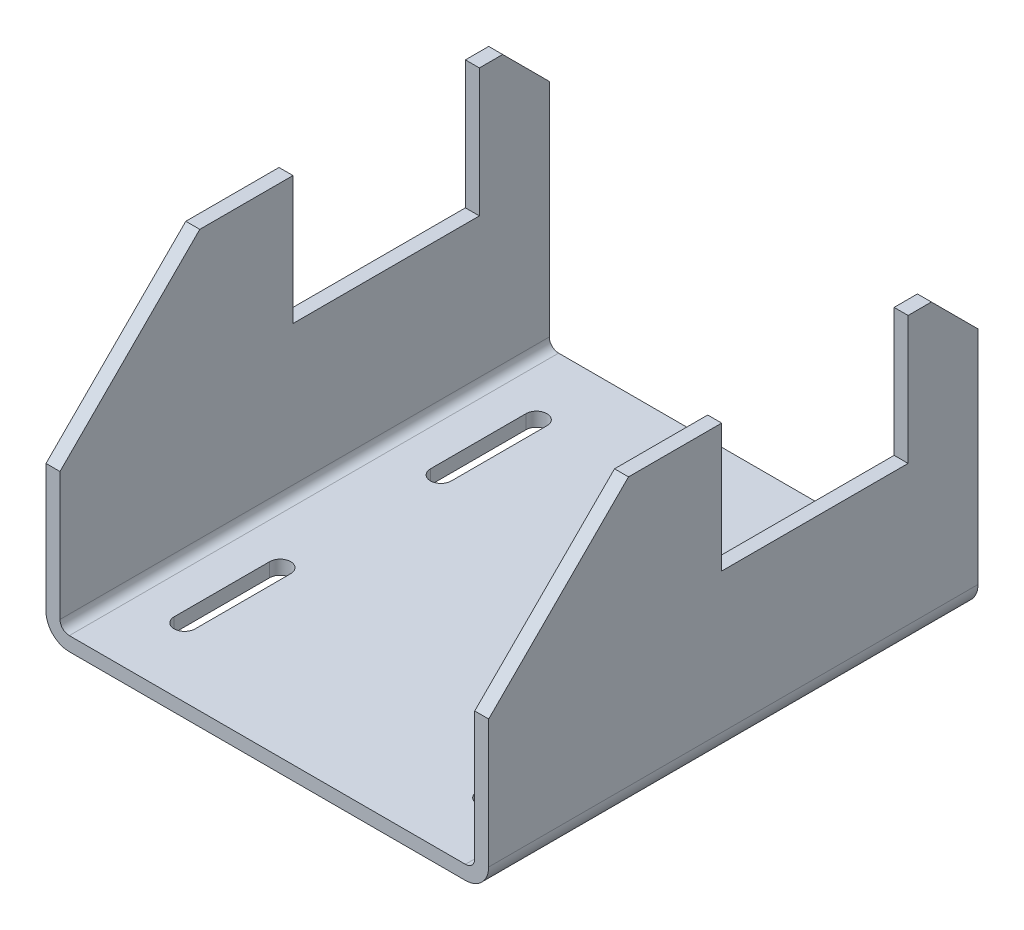
from build123d import *

# Parameters (mm, degrees)
EXTRUDE_1_DEPTH     = 210
CHAMFER_1_SIZE      = 60
CHAMFER_2_SIZE      = 20
CUT_EXTRUDE_1_DEPTH = 417
SKETCH_4_W          = 80
SKETCH_4_H          = 90.775966299
CUT_EXTRUDE_2_DEPTH = 269


with BuildPart() as part:
    # 草图1 → 凸台-拉伸1 (new body)
    with BuildSketch(Plane.XY):
        with BuildLine():
            Line((0, 0), (0, -115))
            ThreePointArc((0, -115), (2.928932188, -122.071067812), (10, -125))
            Line((10, -125), (180, -125))
            ThreePointArc((180, -125), (187.071067812, -122.071067812), (190, -115))
            Line((190, -115), (190, 0))
            Line((190, 0), (184, 0))
            Line((184, 0), (184, -115))
            ThreePointArc((184, -115), (182.828427125, -117.828427125), (180, -119))
            Line((180, -119), (10, -119))
            ThreePointArc((10, -119), (7.171572875, -117.828427125), (6, -115))
            Line((6, -115), (6, 0))
            Line((6, 0), (0, 0))
        make_face()
    extrude(amount=EXTRUDE_1_DEPTH)

    # 倒角1
    chamfer_1_edges = [part.edges().sort_by_distance(p)[0] for p in [
        (187, 0, 210),
        (3, 0, 210),
    ]]
    chamfer(chamfer_1_edges, length=CHAMFER_1_SIZE)

    # 倒角2
    chamfer_2_edges = [part.edges().sort_by_distance(p)[0] for p in [
        (187, 0, 0),
        (3, 0, 0),
    ]]
    chamfer(chamfer_2_edges, length=CHAMFER_2_SIZE)

    # 草图3 → 切除-拉伸1 (cut)
    with BuildSketch(Plane.XZ.offset(125)):
        with BuildLine():
            Line((34.5, 180.5), (34.5, 139.5))
            ThreePointArc((34.5, 139.5), (30, 135), (25.5, 139.5))
            Line((25.5, 139.5), (25.5, 180.5))
            ThreePointArc((25.5, 180.5), (30, 185), (34.5, 180.5))
        make_face()
        with BuildLine():
            Line((164.5, 180.5), (164.5, 139.5))
            ThreePointArc((164.5, 139.5), (160, 135), (155.5, 139.5))
            Line((155.5, 139.5), (155.5, 180.5))
            ThreePointArc((155.5, 180.5), (160, 185), (164.5, 180.5))
        make_face()
        with BuildLine():
            Line((34.5, 70.5), (34.5, 29.5))
            ThreePointArc((34.5, 29.5), (30, 25), (25.5, 29.5))
            Line((25.5, 29.5), (25.5, 70.5))
            ThreePointArc((25.5, 70.5), (30, 75), (34.5, 70.5))
        make_face()
        with BuildLine():
            Line((164.5, 70.5), (164.5, 29.5))
            ThreePointArc((164.5, 29.5), (160, 25), (155.5, 29.5))
            Line((155.5, 29.5), (155.5, 70.5))
            ThreePointArc((155.5, 70.5), (160, 75), (164.5, 70.5))
        make_face()
    extrude(amount=-CUT_EXTRUDE_1_DEPTH, mode=Mode.SUBTRACT)

    # 草图4 → 切除-拉伸2 (cut)
    with BuildSketch(Plane(origin=(190, 0, 0), x_dir=(0, 0, -1), z_dir=(1, 0, 0))):
        with Locations((-70, -9.61201685)):
            Rectangle(SKETCH_4_W, SKETCH_4_H)
    extrude(amount=-CUT_EXTRUDE_2_DEPTH, mode=Mode.SUBTRACT)


solid = part.part
